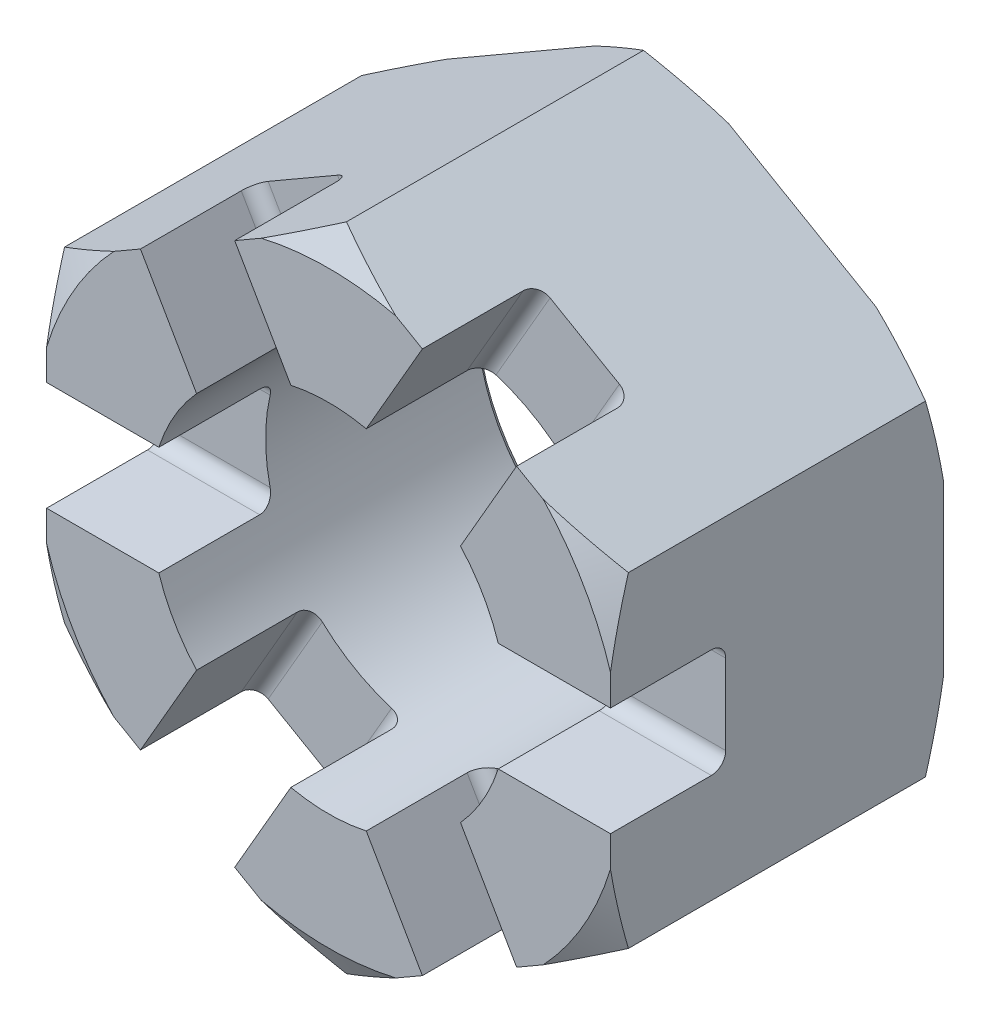
from build123d import *

# Parameters (mm, degrees)
SKETCH_1_R               = 13.9175
EXTRUDE_816_DEPTH        = 26
SKETCH_2_OUTSIDE_W       = 211.19
SKETCH_2_OUTSIDE_H       = 218.002
SKETCH_2_OUTSIDE_R       = 23
CUT_EXTRUDE_1_DEPTH      = 43.511805346
CUT_EXTRUDE_1_DRAFT      = -60
SKETCH_3_OUTSIDE_W       = 211.19
SKETCH_3_OUTSIDE_H       = 218.002
SKETCH_3_OUTSIDE_R       = 23
CUT_EXTRUDE_2_DEPTH      = 43.511805346
CUT_EXTRUDE_2_DRAFT      = -60
CUT_EXTRUDE_3_DEPTH      = 58.111491838
PATTERN_CIRCULAR_1_COUNT = 3
CHAMFER_1_SIZE           = 0.478571429


with BuildPart() as part:
    # 草图1 → Extrude 816 (new body)
    with BuildSketch(Plane.XY):
        Polygon((0, 25.425), (-22.018695891, 12.7125), (-22.018695891, -12.7125), (0, -25.425), (22.018695891, -12.7125), (22.018695891, 12.7125), align=None)
        with Locations(Location((0, 0, 0), (0, 0, 180))):
            Circle(SKETCH_1_R, mode=Mode.SUBTRACT)
    extrude(amount=EXTRUDE_816_DEPTH)


with BuildPart() as cut_extrude_1_tool:
    # 草图2 outside → 切除-拉伸1 (with draft: the straight prism first)
    with BuildSketch(Plane(origin=(0, 0, 0), x_dir=(-1, 0, 0), z_dir=(0, 0, -1))):
        Rectangle(SKETCH_2_OUTSIDE_W, SKETCH_2_OUTSIDE_H)
        Circle(SKETCH_2_OUTSIDE_R, mode=Mode.SUBTRACT)
    extrude(amount=-CUT_EXTRUDE_1_DEPTH)
    # 切除-拉伸1: the draft: its side faces are tilted about the plane it starts from
    cut_extrude_1_sides = [cut_extrude_1_tool.faces().sort_by_distance(p)[0] for p in [
        (0, -109.001, 21.755902673),
        (-105.595, 0, 21.755902673),
        (0, 109.001, 21.755902673),
        (105.595, 0, 21.755902673),
        (23, 0, 21.755902673),
    ]]
    draft(cut_extrude_1_sides, Plane(origin=(0, 0, 0), x_dir=(-1, 0, 0), z_dir=(0, 0, -1)), CUT_EXTRUDE_1_DRAFT)


with BuildPart() as part_1:
    add(part.part)

    # 切除-拉伸1: cut by cut_extrude_1_tool
    add(cut_extrude_1_tool.part, mode=Mode.SUBTRACT)


with BuildPart() as cut_extrude_2_tool:
    # 草图3 outside → 切除-拉伸2 (with draft: the straight prism first)
    with BuildSketch(Plane.XY.offset(26)):
        Rectangle(SKETCH_3_OUTSIDE_W, SKETCH_3_OUTSIDE_H)
        Circle(SKETCH_3_OUTSIDE_R, mode=Mode.SUBTRACT)
    extrude(amount=-CUT_EXTRUDE_2_DEPTH)
    # 切除-拉伸2: the draft: its side faces are tilted about the plane it starts from
    cut_extrude_2_sides = [cut_extrude_2_tool.faces().sort_by_distance(p)[0] for p in [
        (0, -109.001, 4.244097327),
        (105.595, 0, 4.244097327),
        (0, 109.001, 4.244097327),
        (-105.595, 0, 4.244097327),
        (-23, 0, 4.244097327),
    ]]
    draft(cut_extrude_2_sides, Plane.XY.offset(26), CUT_EXTRUDE_2_DRAFT)


with BuildPart() as part_2:
    add(part_1.part)

    # 切除-拉伸2: cut by cut_extrude_2_tool
    add(cut_extrude_2_tool.part, mode=Mode.SUBTRACT)

    # 草图6 → 切除-拉伸3 (cut, through all)
    with BuildSketch(Plane(origin=(22.018695891, 0, 0), x_dir=(0, 0, -1), z_dir=(1, 0, 0))):
        with BuildLine():
            Line((-26, -4.25), (-26, 4.25))
            Line((-26, 4.25), (-18.125, 4.25))
            ThreePointArc((-18.125, 4.25), (-17.329504871, 3.920495129), (-17, 3.125))
            Line((-17, 3.125), (-17, -3.125))
            ThreePointArc((-17, -3.125), (-17.329504871, -3.920495129), (-18.125, -4.25))
            Line((-18.125, -4.25), (-26, -4.25))
        make_face()
    cut_extrude_3 = extrude(amount=-CUT_EXTRUDE_3_DEPTH, mode=Mode.SUBTRACT)

    # 阵列(圆周)1: 切除-拉伸3 ×3 about axis
    pattern_circular_1_axis = Axis((0, 0, 0), (0, 0, 1))
    for i in range(1, PATTERN_CIRCULAR_1_COUNT):
        add(cut_extrude_3.rotate(pattern_circular_1_axis, i * 360 / PATTERN_CIRCULAR_1_COUNT), mode=Mode.SUBTRACT)

    # 倒角1
    chamfer_1_edges = [part_2.edges().sort_by_distance(p)[0] for p in [
        (13.9175, 0, 0),
    ]]
    chamfer(chamfer_1_edges, length=CHAMFER_1_SIZE)


solid = part_2.part
